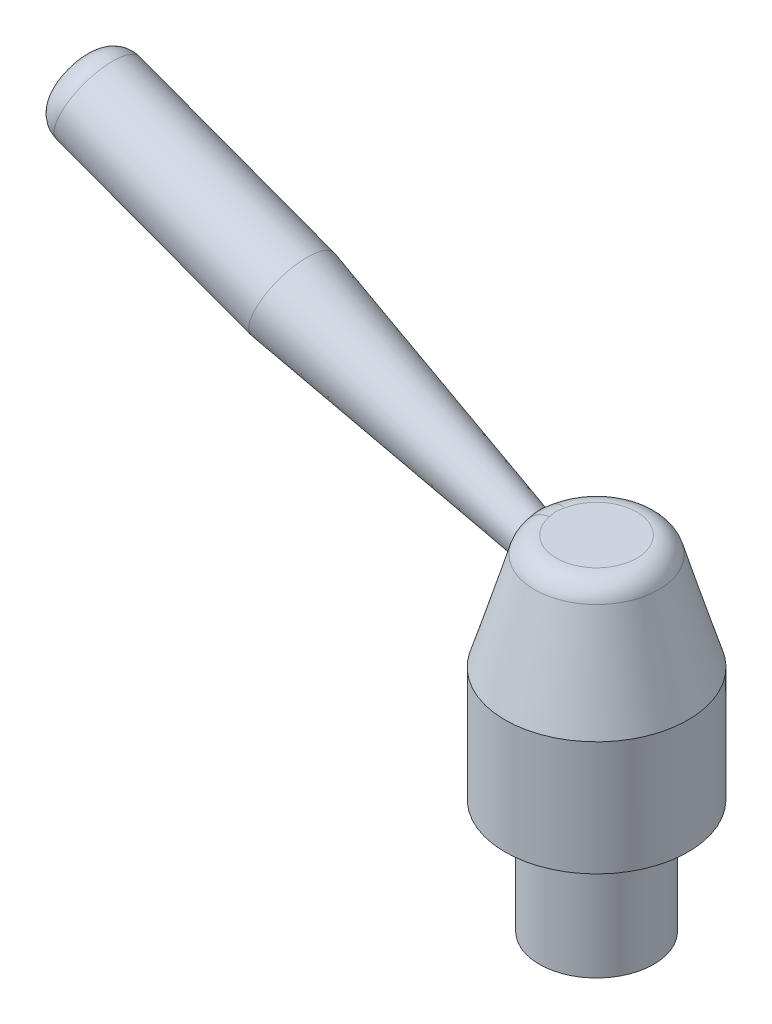
from build123d import *

# Parameters (mm, degrees)
SKETCH4_R           = 5
BOSS_EXTRUDE1_DEPTH = 10
FILLET1_R           = 2


with BuildPart() as part:
    # Sketch2 → Revolve1 (revolve)
    with BuildSketch(Plane.XY):
        Polygon((0, 0), (0, 10), (0, 20), (-5, 20), (-8, 10), (-8, 0), align=None)
    revolve(axis=Axis((0, 20, 0), (0, -1, 0)))

    # Sketch3 → Revolve2 (revolve)
    with BuildSketch(Plane.XY, mode=Mode.PRIVATE) as revolve2_sk:
        Polygon((-45.457291118, 32.007434158), (-46.721063236, 28.616826036), (-27.844496784, 21.581014904), (-4.192388941, 14.958215321), (-3.646298208, 16.423336801), align=None)
    revolve(revolve2_sk.sketch.rotate(Axis((-3.646298208, 16.423336801, 0), (-0.9370274611537507, 0.34925569006639867, 0)), 180), axis=Axis((-3.646298208, 16.423336801, 0), (-0.9370274611537507, 0.34925569006639867, 0)))

    # Sketch4 → Boss-Extrude1 (add)
    with BuildSketch(Plane.XZ):
        Circle(SKETCH4_R)
    extrude(amount=BOSS_EXTRUDE1_DEPTH)

    # Fillet1
    fillet1_edges = [part.edges().sort_by_distance(p)[0] for p in [
        (-46.721063236, 28.616826036, 0),
        (5, 20, 0),
    ]]
    fillet(fillet1_edges, radius=FILLET1_R)


solid = part.part
